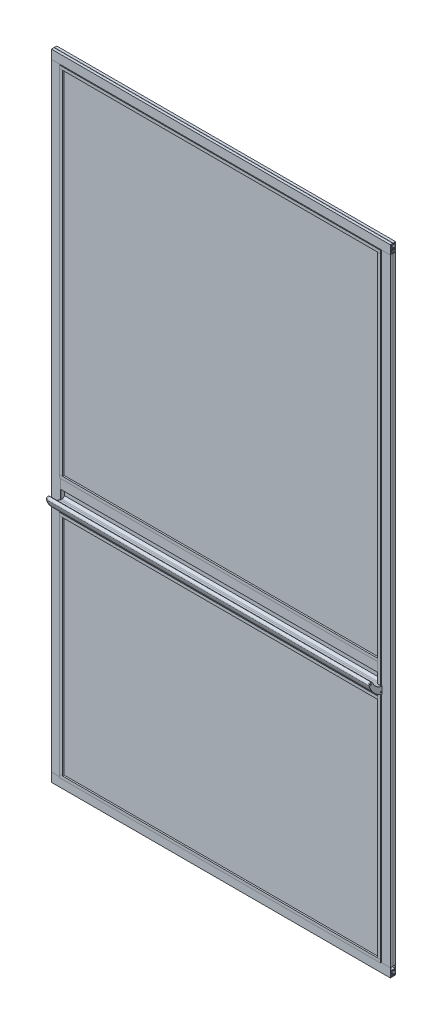
from build123d import *

# Parameters (mm, degrees)
D_XXXXXX_XX_XXXX_XXXX_XXXXXX_XXX_XXXXXXX_DEPTH = 1140
D_XXXXXX_XX_XXXX_XXXX_XXXXXX_XXX_XXX_2_DEPTH   = 1140
D_XXXXXX_XX_XXXX_XXXX_XXXXXX_XXX_XXX_3_DEPTH   = 2138
D_XXXXXX_XX_XXXX_XXXX_XXXXXX_XXX_XXX_5_DEPTH   = 2138
EXTRUDE_2705_DEPTH                             = 1080
EXTRUDE_2952_DEPTH                             = 1080
EXTRUDE_START                                  = 10
EXTRUDE_3223_DEPTH                             = 2056
EXTRUDE_3223_2_DEPTH                           = 2056
SKETCH_2_W                                     = 1072
SKETCH_2_H                                     = 2068
EXTRUDE_3851_DEPTH                             = 17
SKETCH_17_W                                    = 1056
SKETCH_17_H                                    = 2052
EXTRUDE_10_DEPTH                               = 6
EXTRUDE_2_DEPTH                                = 1080
SKETCH_6_R                                     = 2
EXTRUDE_3_DEPTH                                = 3
SKETCH_7_R                                     = 2
EXTRUDE_4_DEPTH                                = 2
SKETCH_8_R                                     = 2
EXTRUDE_5_DEPTH                                = 3
CUT_EXTRUDE_4_DEPTH                            = 1542.282823874
CUT_EXTRUDE_4_DEPTH_BACK                       = 1542.282823874
SKETCH_14_W                                    = 30
SKETCH_14_H                                    = 120
CUT_EXTRUDE_5_DEPTH                            = 1542.282823874
CUT_EXTRUDE_5_DEPTH_BACK                       = 1542.282823874
SKETCH_15_W                                    = 19.3
SKETCH_15_H                                    = 108
CUT_EXTRUDE_6_DEPTH                            = 1533.663284342
CUT_EXTRUDE_6_DEPTH_BACK                       = 1533.663284342
SKETCH_18_W                                    = 6
SKETCH_18_H                                    = 124


with BuildPart() as part:
    # Sketch1 → D_xxxxxx_xx_xxxx_xxxx_xxxxxx_xxx_xxxxxxx (new body)
    with BuildSketch(Plane(origin=(-570, 1068, 0), x_dir=(0, 0, -1), z_dir=(1, 0, 0))):
        with BuildLine():
            Line((-0.5, 0), (-9, 0))
            Line((-9, 0), (-9, -30))
            Line((-9, -30), (-5.9, -30))
            Line((-5.9, -30), (-5.9, -28.5))
            Line((-5.9, -28.5), (-7, -28.5))
            Line((-7, -28.5), (-7, -20))
            Line((-7, -20), (7, -20))
            Line((7, -20), (7, -28.5))
            Line((7, -28.5), (5.9, -28.5))
            Line((5.9, -28.5), (5.9, -30))
            Line((5.9, -30), (9, -30))
            Line((9, -30), (9, 0))
            Line((9, 0), (0.5, 0))
            ThreePointArc((0.5, 0), (0, -0.5), (-0.5, 0))
        make_face()
        with BuildLine():
            Line((-1.341640787, -3), (1.341640786, -3))
            ThreePointArc((1.341640786, -3), (1.799302724, -4.250096987), (1.272792206, -5.472792206))
            ThreePointArc((1.272792206, -5.472792206), (1.272792206, -6.250609665), (2.050609665, -6.250609665))
            ThreePointArc((2.050609665, -6.250609665), (2.853462499, -4.717447359), (2.640075756, -3))
            Line((2.640075756, -3), (7, -3))
            Line((7, -3), (7, -18))
            Line((7, -18), (2.640075756, -18))
            ThreePointArc((2.640075756, -18), (2.853462499, -16.282552641), (2.050609665, -14.749390335))
            ThreePointArc((2.050609665, -14.749390335), (1.272792206, -14.749390335), (1.272792206, -15.527207794))
            ThreePointArc((1.272792206, -15.527207794), (1.799302724, -16.749903013), (1.341640786, -18))
            Line((1.341640786, -18), (-1.341640787, -18))
            ThreePointArc((-1.341640787, -18), (-1.799302724, -16.749903013), (-1.272792206, -15.527207794))
            ThreePointArc((-1.272792206, -15.527207794), (-1.272792206, -14.749390335), (-2.050609665, -14.749390335))
            ThreePointArc((-2.050609665, -14.749390335), (-2.853462499, -16.282552641), (-2.640075756, -18))
            Line((-2.640075756, -18), (-7, -18))
            Line((-7, -18), (-7, -3))
            Line((-7, -3), (-2.640075756, -3))
            ThreePointArc((-2.640075756, -3), (-2.853462499, -4.717447359), (-2.050609665, -6.250609665))
            ThreePointArc((-2.050609665, -6.250609665), (-1.272792206, -6.250609665), (-1.272792206, -5.472792206))
            ThreePointArc((-1.272792206, -5.472792206), (-1.799302724, -4.250096987), (-1.341640787, -3))
        make_face(mode=Mode.SUBTRACT)
    extrude(amount=D_XXXXXX_XX_XXXX_XXXX_XXXXXX_XXX_XXXXXXX_DEPTH)


with BuildPart() as body_2:
    # Sketch1 on segment 2 (carried to segment 2) → D_xxxxxx_xx_xxxx_xxxx_xxxxxx_xxx_xxx 2 (new body)
    with BuildSketch(Plane(origin=(-570, -1068, 0), x_dir=(0, 0, 1), z_dir=(1, 0, 0))):
        with BuildLine():
            Line((-0.5, 0), (-9, 0))
            Line((-9, 0), (-9, -30))
            Line((-9, -30), (-5.9, -30))
            Line((-5.9, -30), (-5.9, -28.5))
            Line((-5.9, -28.5), (-7, -28.5))
            Line((-7, -28.5), (-7, -20))
            Line((-7, -20), (7, -20))
            Line((7, -20), (7, -28.5))
            Line((7, -28.5), (5.9, -28.5))
            Line((5.9, -28.5), (5.9, -30))
            Line((5.9, -30), (9, -30))
            Line((9, -30), (9, 0))
            Line((9, 0), (0.5, 0))
            ThreePointArc((0.5, 0), (0, -0.5), (-0.5, 0))
        make_face()
        with BuildLine():
            Line((-1.341640787, -3), (1.341640786, -3))
            ThreePointArc((1.341640786, -3), (1.799302724, -4.250096987), (1.272792206, -5.472792206))
            ThreePointArc((1.272792206, -5.472792206), (1.272792206, -6.250609665), (2.050609665, -6.250609665))
            ThreePointArc((2.050609665, -6.250609665), (2.853462499, -4.717447359), (2.640075756, -3))
            Line((2.640075756, -3), (7, -3))
            Line((7, -3), (7, -18))
            Line((7, -18), (2.640075756, -18))
            ThreePointArc((2.640075756, -18), (2.853462499, -16.282552641), (2.050609665, -14.749390335))
            ThreePointArc((2.050609665, -14.749390335), (1.272792206, -14.749390335), (1.272792206, -15.527207794))
            ThreePointArc((1.272792206, -15.527207794), (1.799302724, -16.749903013), (1.341640786, -18))
            Line((1.341640786, -18), (-1.341640787, -18))
            ThreePointArc((-1.341640787, -18), (-1.799302724, -16.749903013), (-1.272792206, -15.527207794))
            ThreePointArc((-1.272792206, -15.527207794), (-1.272792206, -14.749390335), (-2.050609665, -14.749390335))
            ThreePointArc((-2.050609665, -14.749390335), (-2.853462499, -16.282552641), (-2.640075756, -18))
            Line((-2.640075756, -18), (-7, -18))
            Line((-7, -18), (-7, -3))
            Line((-7, -3), (-2.640075756, -3))
            ThreePointArc((-2.640075756, -3), (-2.853462499, -4.717447359), (-2.050609665, -6.250609665))
            ThreePointArc((-2.050609665, -6.250609665), (-1.272792206, -6.250609665), (-1.272792206, -5.472792206))
            ThreePointArc((-1.272792206, -5.472792206), (-1.799302724, -4.250096987), (-1.341640787, -3))
        make_face(mode=Mode.SUBTRACT)
    extrude(amount=D_XXXXXX_XX_XXXX_XXXX_XXXXXX_XXX_XXX_2_DEPTH)


with BuildPart() as body_3:
    # Sketch1 on segment 3 (carried to segment 3) → D_xxxxxx_xx_xxxx_xxxx_xxxxxx_xxx_xxx 3 (new body)
    with BuildSketch(Plane(origin=(570, 1069, 0), x_dir=(0, 0, -1), z_dir=(0, -1, 0))):
        with BuildLine():
            Line((-0.5, 0), (-9, 0))
            Line((-9, 0), (-9, -30))
            Line((-9, -30), (-5.9, -30))
            Line((-5.9, -30), (-5.9, -28.5))
            Line((-5.9, -28.5), (-7, -28.5))
            Line((-7, -28.5), (-7, -20))
            Line((-7, -20), (7, -20))
            Line((7, -20), (7, -28.5))
            Line((7, -28.5), (5.9, -28.5))
            Line((5.9, -28.5), (5.9, -30))
            Line((5.9, -30), (9, -30))
            Line((9, -30), (9, 0))
            Line((9, 0), (0.5, 0))
            ThreePointArc((0.5, 0), (0, -0.5), (-0.5, 0))
        make_face()
        with BuildLine():
            Line((-1.341640787, -3), (1.341640786, -3))
            ThreePointArc((1.341640786, -3), (1.799302724, -4.250096987), (1.272792206, -5.472792206))
            ThreePointArc((1.272792206, -5.472792206), (1.272792206, -6.250609665), (2.050609665, -6.250609665))
            ThreePointArc((2.050609665, -6.250609665), (2.853462499, -4.717447359), (2.640075756, -3))
            Line((2.640075756, -3), (7, -3))
            Line((7, -3), (7, -18))
            Line((7, -18), (2.640075756, -18))
            ThreePointArc((2.640075756, -18), (2.853462499, -16.282552641), (2.050609665, -14.749390335))
            ThreePointArc((2.050609665, -14.749390335), (1.272792206, -14.749390335), (1.272792206, -15.527207794))
            ThreePointArc((1.272792206, -15.527207794), (1.799302724, -16.749903013), (1.341640786, -18))
            Line((1.341640786, -18), (-1.341640787, -18))
            ThreePointArc((-1.341640787, -18), (-1.799302724, -16.749903013), (-1.272792206, -15.527207794))
            ThreePointArc((-1.272792206, -15.527207794), (-1.272792206, -14.749390335), (-2.050609665, -14.749390335))
            ThreePointArc((-2.050609665, -14.749390335), (-2.853462499, -16.282552641), (-2.640075756, -18))
            Line((-2.640075756, -18), (-7, -18))
            Line((-7, -18), (-7, -3))
            Line((-7, -3), (-2.640075756, -3))
            ThreePointArc((-2.640075756, -3), (-2.853462499, -4.717447359), (-2.050609665, -6.250609665))
            ThreePointArc((-2.050609665, -6.250609665), (-1.272792206, -6.250609665), (-1.272792206, -5.472792206))
            ThreePointArc((-1.272792206, -5.472792206), (-1.799302724, -4.250096987), (-1.341640787, -3))
        make_face(mode=Mode.SUBTRACT)
    extrude(amount=D_XXXXXX_XX_XXXX_XXXX_XXXXXX_XXX_XXX_3_DEPTH)

    # D_xxxxxx_xx_xxxx_xxxx_xxxxxx_xxx_xxx 3 e
    split(bisect_by=Plane(origin=(570, 1038, 0), x_dir=(1, 0, 0), z_dir=(0, -1, 0)), keep=Keep.TOP)

    # D_xxxxxx_xx_xxxx_xxxx_xxxxxx_xxx_xxx 4
    split(bisect_by=Plane(origin=(570, -1038, 0), x_dir=(-1, 0, 0), z_dir=(0, 1, 0)), keep=Keep.TOP)


with BuildPart() as body_4:
    # Sketch1 on segment 4 (carried to segment 4) → D_xxxxxx_xx_xxxx_xxxx_xxxxxx_xxx_xxx 5 (new body)
    with BuildSketch(Plane(origin=(-570, 1069, 0), x_dir=(0, 0, 1), z_dir=(0, -1, 0))):
        with BuildLine():
            Line((-0.5, 0), (-9, 0))
            Line((-9, 0), (-9, -30))
            Line((-9, -30), (-5.9, -30))
            Line((-5.9, -30), (-5.9, -28.5))
            Line((-5.9, -28.5), (-7, -28.5))
            Line((-7, -28.5), (-7, -20))
            Line((-7, -20), (7, -20))
            Line((7, -20), (7, -28.5))
            Line((7, -28.5), (5.9, -28.5))
            Line((5.9, -28.5), (5.9, -30))
            Line((5.9, -30), (9, -30))
            Line((9, -30), (9, 0))
            Line((9, 0), (0.5, 0))
            ThreePointArc((0.5, 0), (0, -0.5), (-0.5, 0))
        make_face()
        with BuildLine():
            Line((-1.341640787, -3), (1.341640786, -3))
            ThreePointArc((1.341640786, -3), (1.799302724, -4.250096987), (1.272792206, -5.472792206))
            ThreePointArc((1.272792206, -5.472792206), (1.272792206, -6.250609665), (2.050609665, -6.250609665))
            ThreePointArc((2.050609665, -6.250609665), (2.853462499, -4.717447359), (2.640075756, -3))
            Line((2.640075756, -3), (7, -3))
            Line((7, -3), (7, -18))
            Line((7, -18), (2.640075756, -18))
            ThreePointArc((2.640075756, -18), (2.853462499, -16.282552641), (2.050609665, -14.749390335))
            ThreePointArc((2.050609665, -14.749390335), (1.272792206, -14.749390335), (1.272792206, -15.527207794))
            ThreePointArc((1.272792206, -15.527207794), (1.799302724, -16.749903013), (1.341640786, -18))
            Line((1.341640786, -18), (-1.341640787, -18))
            ThreePointArc((-1.341640787, -18), (-1.799302724, -16.749903013), (-1.272792206, -15.527207794))
            ThreePointArc((-1.272792206, -15.527207794), (-1.272792206, -14.749390335), (-2.050609665, -14.749390335))
            ThreePointArc((-2.050609665, -14.749390335), (-2.853462499, -16.282552641), (-2.640075756, -18))
            Line((-2.640075756, -18), (-7, -18))
            Line((-7, -18), (-7, -3))
            Line((-7, -3), (-2.640075756, -3))
            ThreePointArc((-2.640075756, -3), (-2.853462499, -4.717447359), (-2.050609665, -6.250609665))
            ThreePointArc((-2.050609665, -6.250609665), (-1.272792206, -6.250609665), (-1.272792206, -5.472792206))
            ThreePointArc((-1.272792206, -5.472792206), (-1.799302724, -4.250096987), (-1.341640787, -3))
        make_face(mode=Mode.SUBTRACT)
    extrude(amount=D_XXXXXX_XX_XXXX_XXXX_XXXXXX_XXX_XXX_5_DEPTH)

    # D_xxxxxx_xx_xxxx_xxxx_xxxxxx_xxx_xxx 5 e
    split(bisect_by=Plane(origin=(-570, 1038, 0), x_dir=(1, 0, 0), z_dir=(0, -1, 0)), keep=Keep.TOP)

    # D_xxxxxx_xx_xxxx_xxxx_xxxxxx_xxx_xxx 6
    split(bisect_by=Plane(origin=(-570, -1038, 0), x_dir=(-1, 0, 0), z_dir=(0, 1, 0)), keep=Keep.TOP)


with BuildPart() as body_5:
    # 草图10 → Extrude 2705 (new body)
    with BuildSketch(Plane(origin=(-540, 0, 0), x_dir=(0, 0, -1), z_dir=(1, 0, 0))):
        Polygon((12.7, 1036), (12.7, 1028), (18.2, 1028), (18.2, 1038), (6, 1038), (6, 1046), (4.2, 1046), (4.2, 1038.000000001), (-4.1, 1038), (-4.1, 1046), (-5.9, 1046), (-5.9, 1038), (-11.8, 1038), (-11.8, 1028), (-6.6, 1028), (-6.6, 1036), align=None)
    extrude(amount=EXTRUDE_2705_DEPTH)


with BuildPart() as body_6:
    # 草图11 → Extrude 2952 (new body)
    with BuildSketch(Plane(origin=(-540, 0, 0), x_dir=(0, 0, -1), z_dir=(1, 0, 0))):
        Polygon((12.7, -1036), (12.7, -1028), (18.2, -1028), (18.2, -1038), (6, -1038), (6, -1046), (4.2, -1046), (4.2, -1038.000000001), (-4.1, -1038), (-4.1, -1046), (-5.9, -1046), (-5.9, -1038), (-11.8, -1038), (-11.8, -1028), (-6.6, -1028), (-6.6, -1036), align=None)
    extrude(amount=EXTRUDE_2952_DEPTH)


with BuildPart() as body_7:
    # 草图12 → Extrude 3223 (new body)
    with BuildSketch(Plane(origin=(0, -1038, 0), x_dir=(1, 0, 0), z_dir=(0, 1, 0)).offset(EXTRUDE_START)):
        Polygon((-538, 12.7), (-530, 12.7), (-530, 18.2), (-540, 18.2), (-540, 6), (-548, 6), (-548, 4.2), (-540.000000001, 4.2), (-540, -4.1), (-548, -4.1), (-548, -5.9), (-540, -5.9), (-540, -11.8), (-530, -11.8), (-530, -6.6), (-538, -6.6), align=None)
    extrude(amount=EXTRUDE_3223_DEPTH)

    # 草图14 → 切除-拉伸4 (cut, two sides: drawn at the far end of the back side and taken through both)
    with BuildSketch(Plane.ZY.offset(540).offset(-CUT_EXTRUDE_4_DEPTH_BACK)):
        with Locations((-3.2, -215)):
            Rectangle(SKETCH_14_W, SKETCH_14_H)
    extrude(amount=CUT_EXTRUDE_4_DEPTH + CUT_EXTRUDE_4_DEPTH_BACK, mode=Mode.SUBTRACT)


with BuildPart() as body_8:
    # 草图12 → Extrude 3223 2 (new body)
    with BuildSketch(Plane(origin=(0, -1038, 0), x_dir=(1, 0, 0), z_dir=(0, 1, 0)).offset(EXTRUDE_START)):
        Polygon((538, 12.7), (530, 12.7), (530, 18.2), (540, 18.2), (540, 6), (548, 6), (548, 4.2), (540.000000001, 4.2), (540, -4.1), (548, -4.1), (548, -5.9), (540, -5.9), (540, -11.8), (530, -11.8), (530, -6.6), (538, -6.6), align=None)
    extrude(amount=EXTRUDE_3223_2_DEPTH)


with BuildPart() as body_9:
    # 草图2 → Extrude 3851 (new body)
    with BuildSketch(Plane.XY.offset(6.6)):
        Rectangle(SKETCH_2_W, SKETCH_2_H)
    extrude(amount=-EXTRUDE_3851_DEPTH)

    # 草图15 → 切除-拉伸5 (cut, two sides: drawn at the far end of the back side and taken through both)
    with BuildSketch(Plane.ZY.offset(540).offset(-CUT_EXTRUDE_5_DEPTH_BACK)):
        with Locations((-3.05, -215)):
            Rectangle(SKETCH_15_W, SKETCH_15_H)
    extrude(amount=CUT_EXTRUDE_5_DEPTH + CUT_EXTRUDE_5_DEPTH_BACK, mode=Mode.SUBTRACT)


with BuildPart() as body_10:
    # 草图17 → 凸台-拉伸10 (new body)
    with BuildSketch(Plane(origin=(0, 0, -10.4), x_dir=(-1, 0, 0), z_dir=(0, 0, -1))):
        Rectangle(SKETCH_17_W, SKETCH_17_H)
    extrude(amount=EXTRUDE_10_DEPTH)

    # 草图18 → 切除-拉伸6 (cut, two sides: drawn at the far end of the back side and taken through both)
    with BuildSketch(Plane.ZY.offset(528).offset(-CUT_EXTRUDE_6_DEPTH_BACK)):
        with Locations((-13.4, -215)):
            Rectangle(SKETCH_18_W, SKETCH_18_H)
    extrude(amount=CUT_EXTRUDE_6_DEPTH + CUT_EXTRUDE_6_DEPTH_BACK, mode=Mode.SUBTRACT)


with BuildPart() as body_11:
    # 草图4 → 凸台-拉伸2 (new body)
    with BuildSketch(Plane.ZY.offset(-540)):
        with BuildLine():
            Line((2.857553645, -197.108927406), (6.704462631, -195.385112329))
            ThreePointArc((6.704462631, -195.385112329), (6.919661361, -195.200645134), (7, -194.928828391))
            Line((7, -194.928828391), (7, -192.952423581))
            ThreePointArc((7, -192.952423581), (6.121320344, -190.831103238), (4, -189.952423581))
            Line((4, -189.952423581), (-4, -189.952423581))
            ThreePointArc((-4, -189.952423581), (-4.707106781, -190.2453168), (-5, -190.952423581))
            Line((-5, -190.952423581), (-5, -199.086015321))
            ThreePointArc((-5, -199.086015321), (-4.543633488, -199.925338042), (-3.591074738, -199.998583198))
            Line((-3.591074738, -199.998583198), (-3.347907918, -199.889619187))
            ThreePointArc((-3.347907918, -199.889619187), (-3.194897044, -199.885245411), (-3.08360929, -199.99034771))
            Line((-3.08360929, -199.99034771), (-2.895538614, -200.410050952))
            ThreePointArc((-2.895538614, -200.410050952), (-2.8816414, -200.529556054), (-2.938818386, -200.635411588))
            Line((-2.938818386, -200.635411588), (-3.678508693, -201.352733376))
            Line((-3.678508693, -201.352733376), (-3.596723641, -201.535246951))
            Line((-3.596723641, -201.535246951), (-3.140439702, -201.33078432))
            ThreePointArc((-3.140439702, -201.33078432), (-2.941801607, -201.350985338), (-2.859622684, -201.532951814))
            Line((-2.859622684, -201.532951814), (-3.131422947, -204.285427902))
            Line((-3.131422947, -204.285427902), (-5, -205.122744643))
            Line((-5, -205.122744643), (-5, -224.876431855))
            ThreePointArc((-5, -224.876431855), (-1.310885546, -228.990696117), (4, -230.517532911))
            Line((4, -230.517532911), (9, -230.517532911))
            ThreePointArc((9, -230.517532911), (29.001605349, -222.801616047), (41.658705692, -205.498512265))
            ThreePointArc((41.658705692, -205.498512265), (49.190680956, -202.177818295), (52.949400099, -209.50104779))
            ThreePointArc((52.949400099, -209.50104779), (36.94100116, -236.960097621), (10.522889115, -254.633569556))
            Line((10.522889115, -254.633569556), (9, -254.633569556))
            Line((9, -254.633569556), (9, -265))
            Line((9, -265), (5.9, -265))
            Line((5.9, -265), (5.9, -263.5))
            Line((5.9, -263.5), (7, -263.5))
            Line((7, -263.5), (7, -255))
            Line((7, -255), (-7, -255))
            Line((-7, -255), (-7, -263.5))
            Line((-7, -263.5), (-5.9, -263.5))
            Line((-5.9, -263.5), (-5.9, -265))
            Line((-5.9, -265), (-9, -265))
            Line((-9, -265), (-9, -255))
            Line((-9, -255), (-8.5, -254.5))
            Line((-8.5, -254.5), (-8.5, -252.5))
            Line((-8.5, -252.5), (-9, -252))
            Line((-9, -252), (-9, -178))
            Line((-9, -178), (-8.5, -177.5))
            Line((-8.5, -177.5), (-8.5, -175.5))
            Line((-8.5, -175.5), (-9, -175))
            Line((-9, -175), (-9, -165))
            Line((-9, -165), (-5.9, -165))
            Line((-5.9, -165), (-5.9, -166.5))
            Line((-5.9, -166.5), (-7, -166.5))
            Line((-7, -166.5), (-7, -175))
            Line((-7, -175), (7, -175))
            Line((7, -175), (7, -166.5))
            Line((7, -166.5), (5.9, -166.5))
            Line((5.9, -166.5), (5.9, -165))
            Line((5.9, -165), (9, -165))
            Line((9, -165), (9, -198.849289471))
            Line((9, -198.849289471), (6.9068237, -199.78725002))
            Line((6.9068237, -199.78725002), (5.994255823, -200.196175282))
            Line((5.994255823, -200.196175282), (3.759062035, -198.567093108))
            ThreePointArc((3.759062035, -198.567093108), (3.677947451, -198.384649697), (3.795076163, -198.222952329))
            Line((3.795076163, -198.222952329), (4.251360101, -198.018489698))
            Line((4.251360101, -198.018489698), (4.169575049, -197.835976122))
            Line((4.169575049, -197.835976122), (3.141897681, -197.910618755))
            ThreePointArc((3.141897681, -197.910618755), (3.024838296, -197.882839225), (2.944895799, -197.792929275))
            Line((2.944895799, -197.792929275), (2.756825122, -197.373226034))
            ThreePointArc((2.756825122, -197.373226034), (2.752451346, -197.220215159), (2.857553645, -197.108927406))
        make_face()
        with BuildLine():
            Line((-0.591607978, -252), (0.591607978, -252))
            ThreePointArc((0.591607978, -252), (1.754528537, -250.702031856), (1.272792206, -249.027207794))
            ThreePointArc((1.272792206, -249.027207794), (1.272792206, -248.249390335), (2.050609665, -248.249390335))
            ThreePointArc((2.050609665, -248.249390335), (2.8908371, -250.069650561), (2.349468025, -252))
            Line((2.349468025, -252), (7, -252))
            Line((7, -252), (7, -232.517532911))
            Line((7, -232.517532911), (4, -232.517532911))
            ThreePointArc((4, -232.517532911), (-1.098439293, -231.380585741), (-5.230769231, -228.185185708))
            ThreePointArc((-5.230769231, -228.185185708), (-6.33968311, -227.883616831), (-7, -228.824156774))
            Line((-7, -228.824156774), (-7, -252))
            Line((-7, -252), (-2.349468025, -252))
            ThreePointArc((-2.349468025, -252), (-2.890837099, -250.069650561), (-2.050609666, -248.249390335))
            ThreePointArc((-2.050609666, -248.249390335), (-1.272792206, -248.249390335), (-1.272792206, -249.027207794))
            ThreePointArc((-1.272792206, -249.027207794), (-1.754528537, -250.702031855), (-0.591607978, -252))
        make_face(mode=Mode.SUBTRACT)
        with BuildLine():
            Line((-2.349468025, -178), (-7, -178))
            Line((-7, -178), (-7, -187.952423581))
            Line((-7, -187.952423581), (7, -187.952423581))
            Line((7, -187.952423581), (7, -178))
            Line((7, -178), (2.349468025, -178))
            ThreePointArc((2.349468025, -178), (2.890837099, -179.930349439), (2.050609665, -181.750609665))
            ThreePointArc((2.050609665, -181.750609665), (1.272792206, -181.750609665), (1.272792206, -180.972792206))
            ThreePointArc((1.272792206, -180.972792206), (1.754528537, -179.297968144), (0.591607978, -178))
            Line((0.591607978, -178), (-0.591607978, -178))
            ThreePointArc((-0.591607978, -178), (-1.754528537, -179.297968144), (-1.272792206, -180.972792206))
            ThreePointArc((-1.272792206, -180.972792206), (-1.272792206, -181.750609665), (-2.050609665, -181.750609665))
            ThreePointArc((-2.050609665, -181.750609665), (-2.8908371, -179.930349439), (-2.349468025, -178))
        make_face(mode=Mode.SUBTRACT)
        with BuildLine():
            Line((47.990278547, -210.512974914), (49.42470127, -210.93826723))
            ThreePointArc((49.42470127, -210.93826723), (49.72344908, -211.181787003), (49.760223756, -211.565453207))
            ThreePointArc((49.760223756, -211.565453207), (37.064728814, -234.546306856), (16.273739662, -250.57846193))
            ThreePointArc((16.273739662, -250.57846193), (15.889893701, -250.600604766), (15.603815834, -250.34372448))
            Line((15.603815834, -250.34372448), (14.904952734, -248.876313524))
            ThreePointArc((14.904952734, -248.876313524), (16.389996434, -247.529474766), (16.646469065, -245.541120868))
            ThreePointArc((16.646469065, -245.541120868), (15.98776331, -245.127470377), (15.574112819, -245.786176132))
            ThreePointArc((15.574112819, -245.786176132), (12.86209147, -247.711531202), (13.418348531, -244.432410889))
            ThreePointArc((13.418348531, -244.432410889), (13.831999022, -243.773705134), (13.173293267, -243.360054644))
            ThreePointArc((13.173293267, -243.360054644), (11.493703581, -244.45472716), (10.925592049, -246.377376042))
            Line((10.925592049, -246.377376042), (9.5, -246.377376042))
            ThreePointArc((9.5, -246.377376042), (9.146446609, -246.230929432), (9, -245.877376042))
            Line((9, -245.877376042), (9, -232.025929779))
            ThreePointArc((9, -232.025929779), (28.875214056, -224.716759873), (42.854511276, -208.809926508))
            ThreePointArc((42.854511276, -208.809926508), (43.15129036, -208.559946567), (43.537497896, -208.597516964))
            Line((43.537497896, -208.597516964), (44.790550315, -209.274708837))
            ThreePointArc((44.790550315, -209.274708837), (45.415980474, -209.180714504), (45.539471562, -208.560434108))
            ThreePointArc((45.539471562, -208.560434108), (47.83577205, -206.154388388), (47.913373649, -209.479449279))
            ThreePointArc((47.913373649, -209.479449279), (47.587164388, -210.023346665), (47.990278547, -210.512974914))
        make_face(mode=Mode.SUBTRACT)
    extrude(amount=EXTRUDE_2_DEPTH)


with BuildPart() as body_12:
    # 草图6 → 凸台-拉伸3 (new body)
    with BuildSketch(Plane.ZY.offset(540)):
        with BuildLine():
            Line((9.5, -254.633569556), (10.522889115, -254.633569556))
            ThreePointArc((10.522889115, -254.633569556), (36.94100116, -236.960097621), (52.949400099, -209.50104779))
            ThreePointArc((52.949400099, -209.50104779), (49.190680956, -202.177818295), (41.658705691, -205.498512265))
            ThreePointArc((41.658705691, -205.498512265), (29.200353014, -222.648317686), (9.5, -230.472796488))
            Line((9.5, -230.472796488), (9.5, -254.633569556))
        make_face()
        with Locations((47.185930191, -207.832990651)):
            Circle(SKETCH_6_R, mode=Mode.SUBTRACT)
        with Locations((13.819348054, -246.187175655)):
            Circle(SKETCH_6_R, mode=Mode.SUBTRACT)
    extrude(amount=EXTRUDE_3_DEPTH)


with BuildPart() as body_13:
    # 草图7 → 凸台-拉伸4 (new body)
    with BuildSketch(Plane.ZY.offset(540)):
        Polygon((-5.7, -178), (-5.7, -189.952423581), (-3.7, -189.952423581), (-3.7, -199.952423581), (-5.7, -199.952423581), (-5.7, -252), (-3.7, -254), (3.7, -254), (5.7, -252), (5.7, -199.952423581), (3.7, -199.952423581), (3.7, -189.952423581), (5.7, -189.952423581), (5.7, -178), (3.7, -176), (-3.7, -176), align=None)
        with Locations((0, -179.7)):
            Circle(SKETCH_7_R, mode=Mode.SUBTRACT)
        with Locations((0, -250.3)):
            Circle(SKETCH_7_R, mode=Mode.SUBTRACT)
    extrude(amount=EXTRUDE_4_DEPTH)


with BuildPart() as body_14:
    # 草图8 → 凸台-拉伸5 (new body)
    with BuildSketch(Plane.ZY.offset(542)):
        Polygon((-6.7, -178), (-6.7, -189.952423581), (-3.7, -189.952423581), (-3.7, -199.952423581), (-6.7, -199.952423581), (-6.7, -252), (-4.7, -254), (4.7, -254), (6.7, -252), (6.7, -199.952423581), (3.7, -199.952423581), (3.7, -189.952423581), (6.7, -189.952423581), (6.7, -178), (4.7, -176), (-4.7, -176), align=None)
        with Locations((0, -179.7)):
            Circle(SKETCH_8_R, mode=Mode.SUBTRACT)
        with Locations((0, -250.3)):
            Circle(SKETCH_8_R, mode=Mode.SUBTRACT)
    extrude(amount=EXTRUDE_5_DEPTH)


with BuildPart() as body_15:
    # 镜向1: mirrored copy
    add(body_12.part.mirror(Plane(origin=(0, 0, 0), x_dir=(0, 0, 1), z_dir=(1, 0, 0))))


with BuildPart() as body_16:
    # Mirror 1 2: mirrored copy
    add(body_13.part.mirror(Plane(origin=(0, 0, 0), x_dir=(0, 0, 1), z_dir=(1, 0, 0))))


with BuildPart() as body_17:
    # Mirror 1 3: mirrored copy
    add(body_14.part.mirror(Plane(origin=(0, 0, 0), x_dir=(0, 0, 1), z_dir=(1, 0, 0))))


with BuildPart() as body_18:
    # 镜向2: mirrored copy
    add(body_5.part.mirror(Plane(origin=(0, 436.5, 0), x_dir=(0, 0, 1), z_dir=(0, -1, 0))))


with BuildPart() as body_19:
    # 镜向3: mirrored copy
    add(body_6.part.mirror(Plane(origin=(0, -651.5, 0), x_dir=(0, 0, 1), z_dir=(0, -1, 0))))


with BuildPart() as cut_extrude_4_piece_1:
    # of the separate pieces the step leaves, piece 1, a body of its own (cut_extrude_4_pieces)
    add(body_7.part.solids().sort_by_distance((-538, -155, -12.7))[0])


with BuildPart() as cut_extrude_4_piece_2:
    # of the separate pieces the step leaves, piece 2, a body of its own (cut_extrude_4_pieces)
    add(body_7.part.solids().sort_by_distance((-538, -1028, -12.7))[0])


with BuildPart() as cut_extrude_5_piece_1:
    # of the separate pieces the step leaves, piece 1, a body of its own (cut_extrude_5_pieces)
    add(body_9.part.solids().sort_by_distance((-536, 1034, 6.6))[0])


with BuildPart() as cut_extrude_5_piece_2:
    # of the separate pieces the step leaves, piece 2, a body of its own (cut_extrude_5_pieces)
    add(body_9.part.solids().sort_by_distance((-536, -1034, 6.6))[0])


with BuildPart() as cut_extrude_6_piece_1:
    # of the separate pieces the step leaves, piece 1, a body of its own (cut_extrude_6_pieces)
    add(body_10.part.solids().sort_by_distance((528, 1026, -10.4))[0])


with BuildPart() as cut_extrude_6_piece_2:
    # of the separate pieces the step leaves, piece 2, a body of its own (cut_extrude_6_pieces)
    add(body_10.part.solids().sort_by_distance((528, -1026, -10.4))[0])


solid = Compound([part.part, body_2.part, body_3.part, body_4.part, body_5.part, body_6.part, body_8.part, body_11.part, body_12.part, body_13.part, body_14.part, body_15.part, body_16.part, body_17.part, body_18.part, body_19.part, cut_extrude_4_piece_1.part, cut_extrude_4_piece_2.part, cut_extrude_5_piece_1.part, cut_extrude_5_piece_2.part, cut_extrude_6_piece_1.part, cut_extrude_6_piece_2.part])
